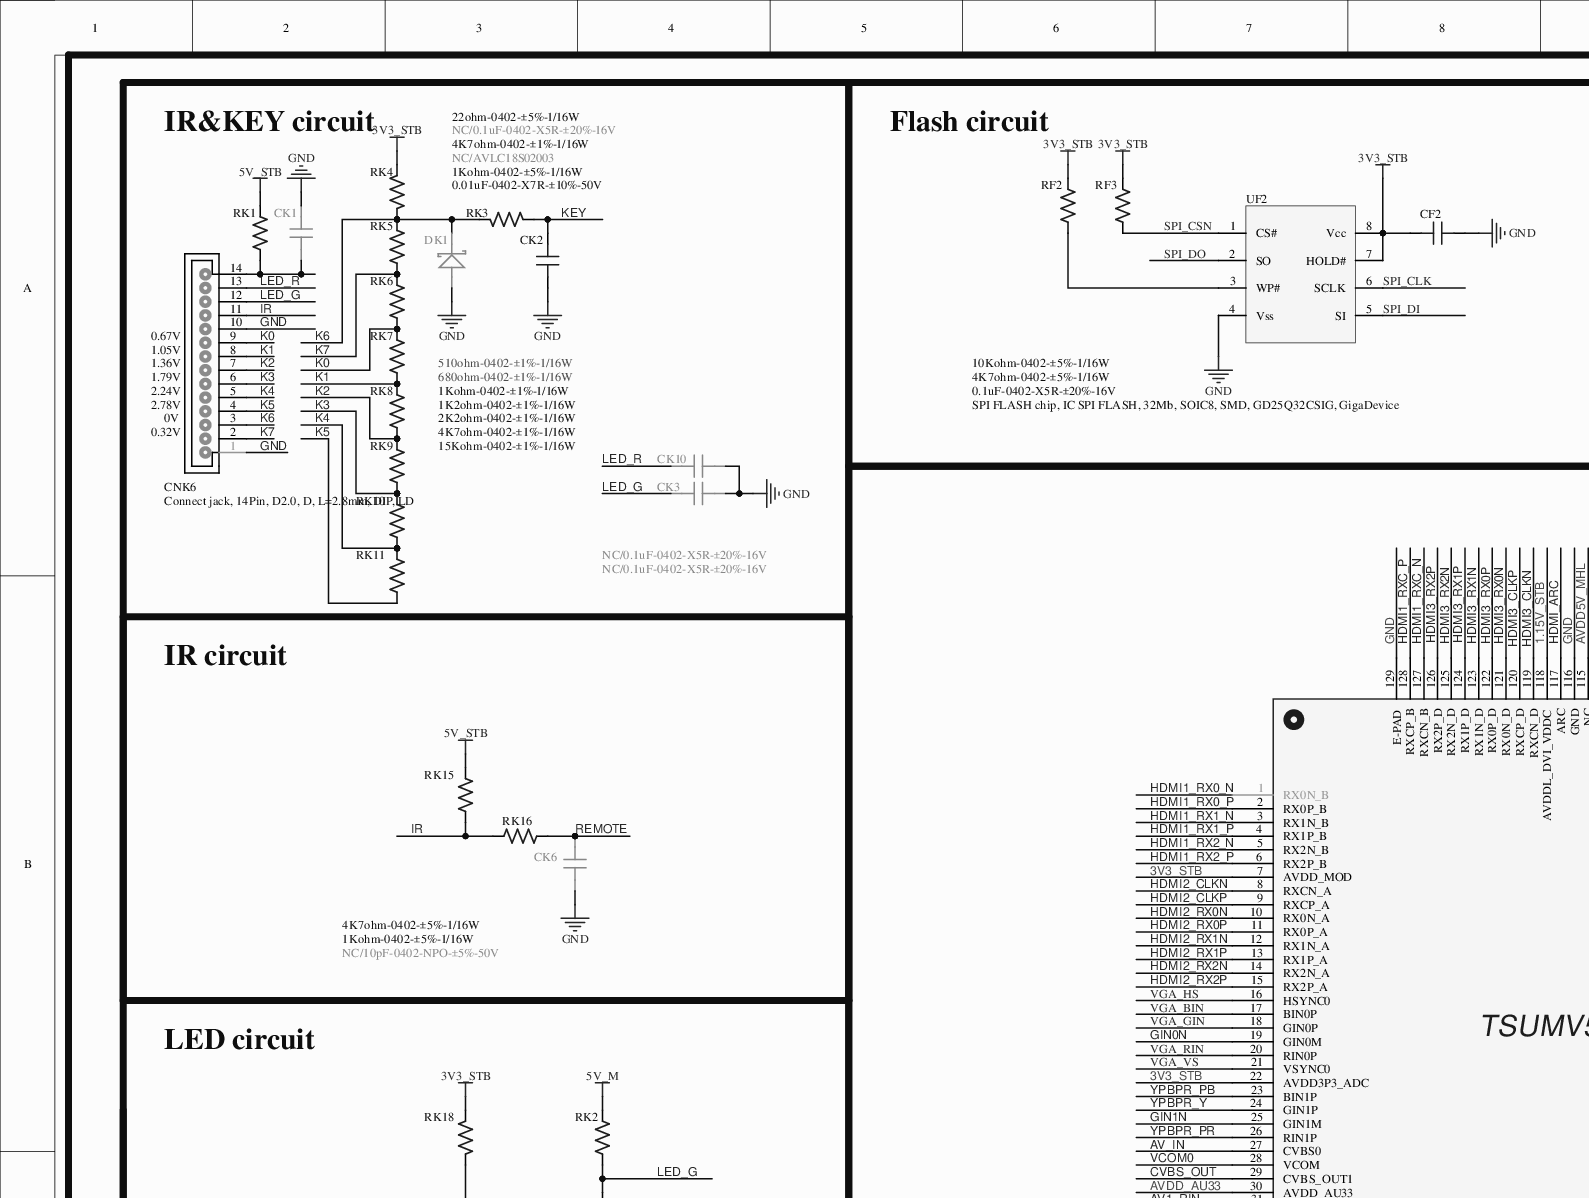
[diagram p0: MISC84277-8.SchDoc, top left]
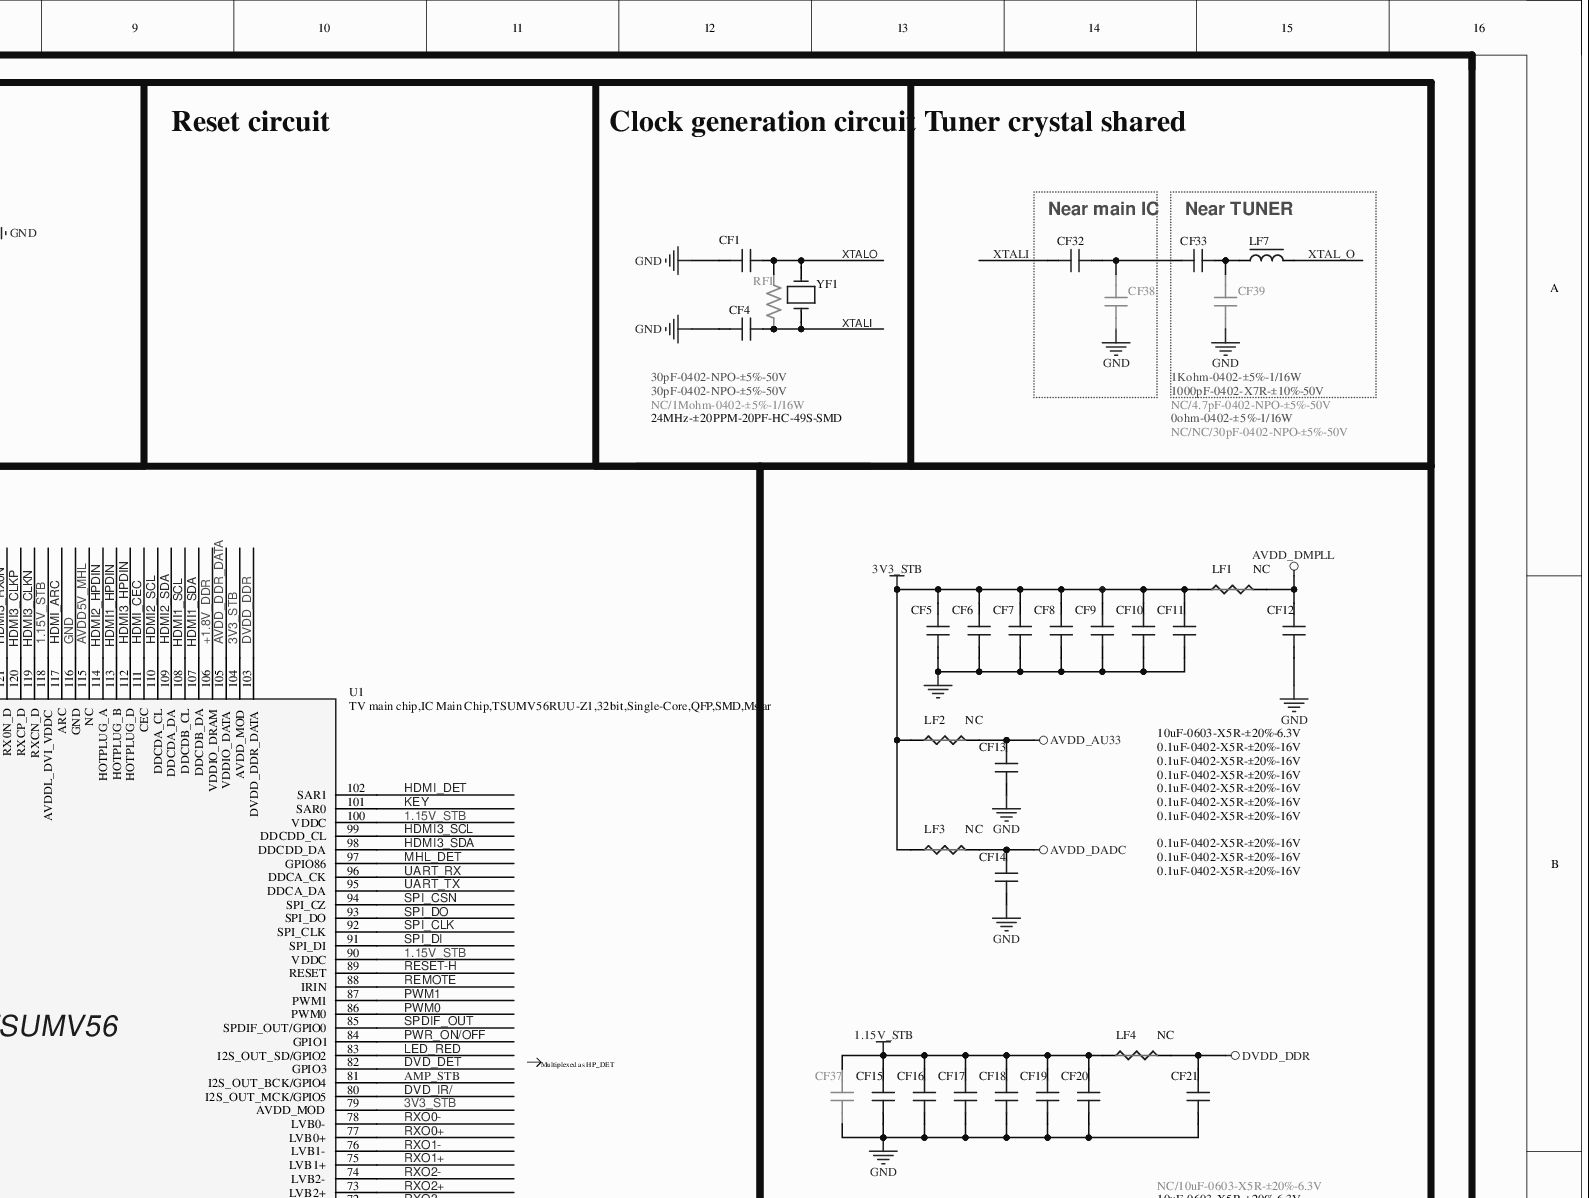
[diagram p1: MISC84277-8.SchDoc, top right]
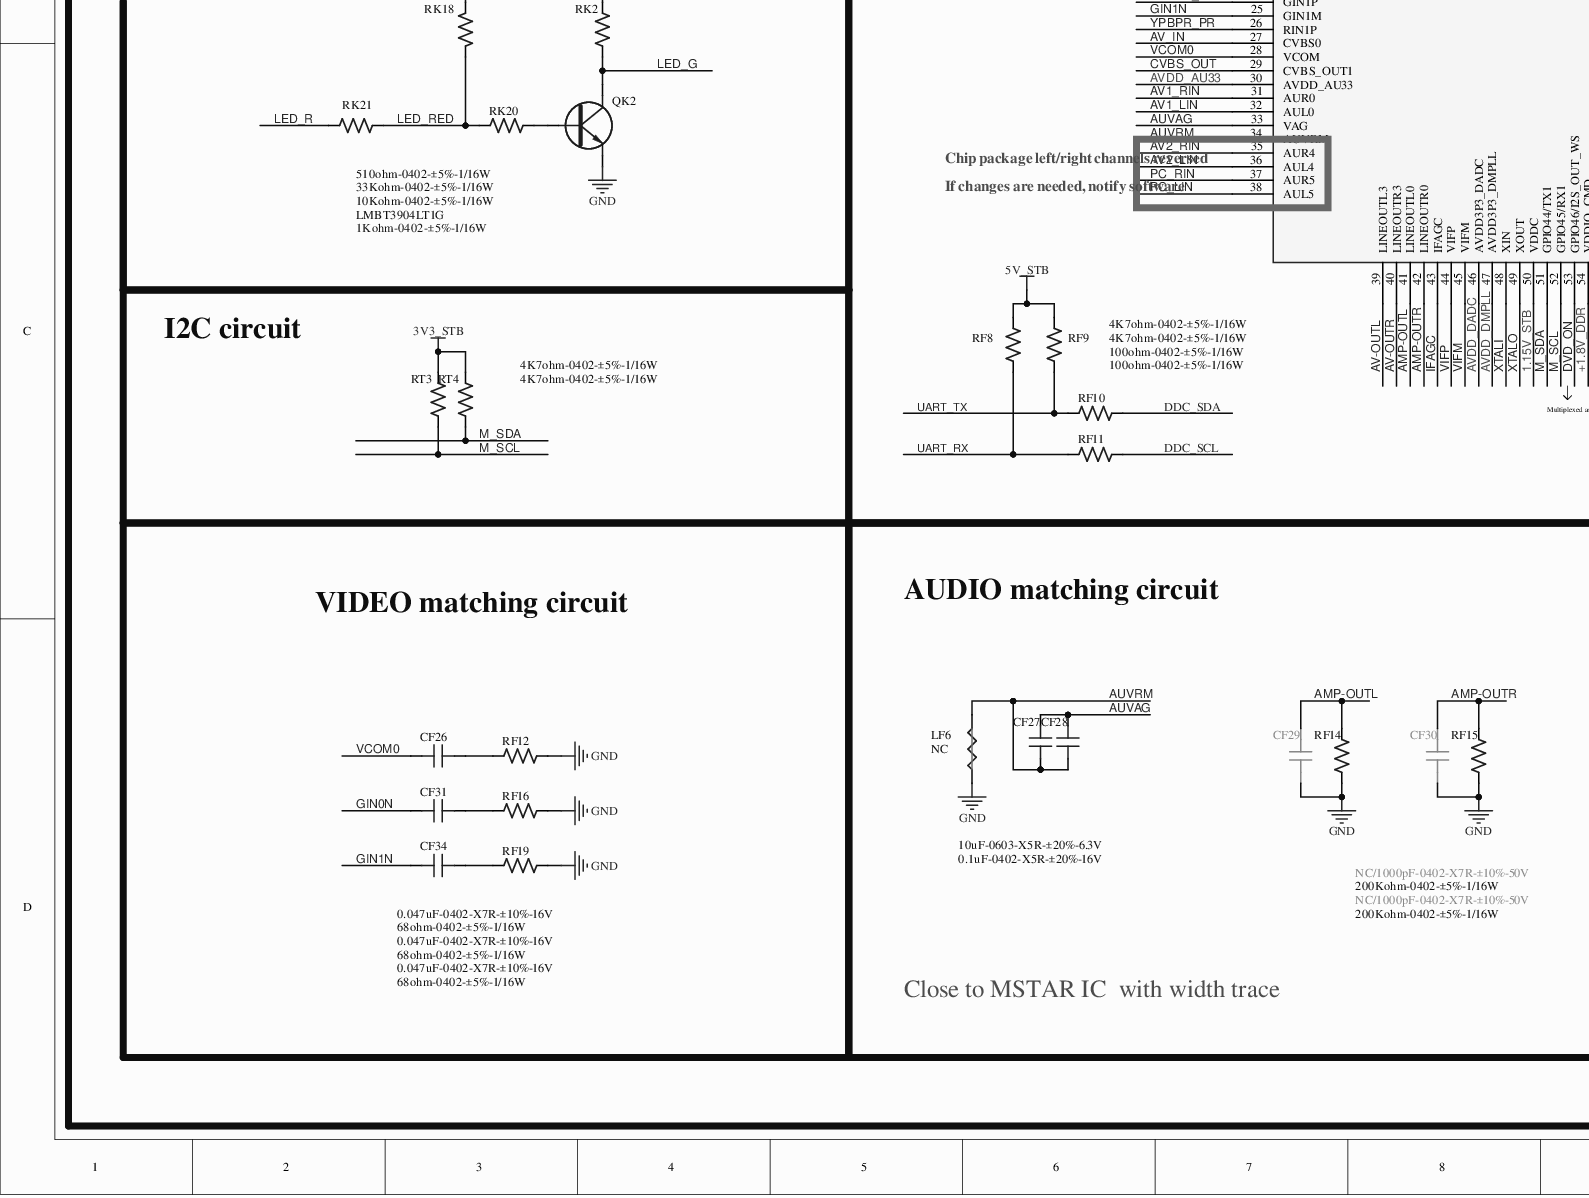
[diagram p2: MISC84277-8.SchDoc, bottom left]
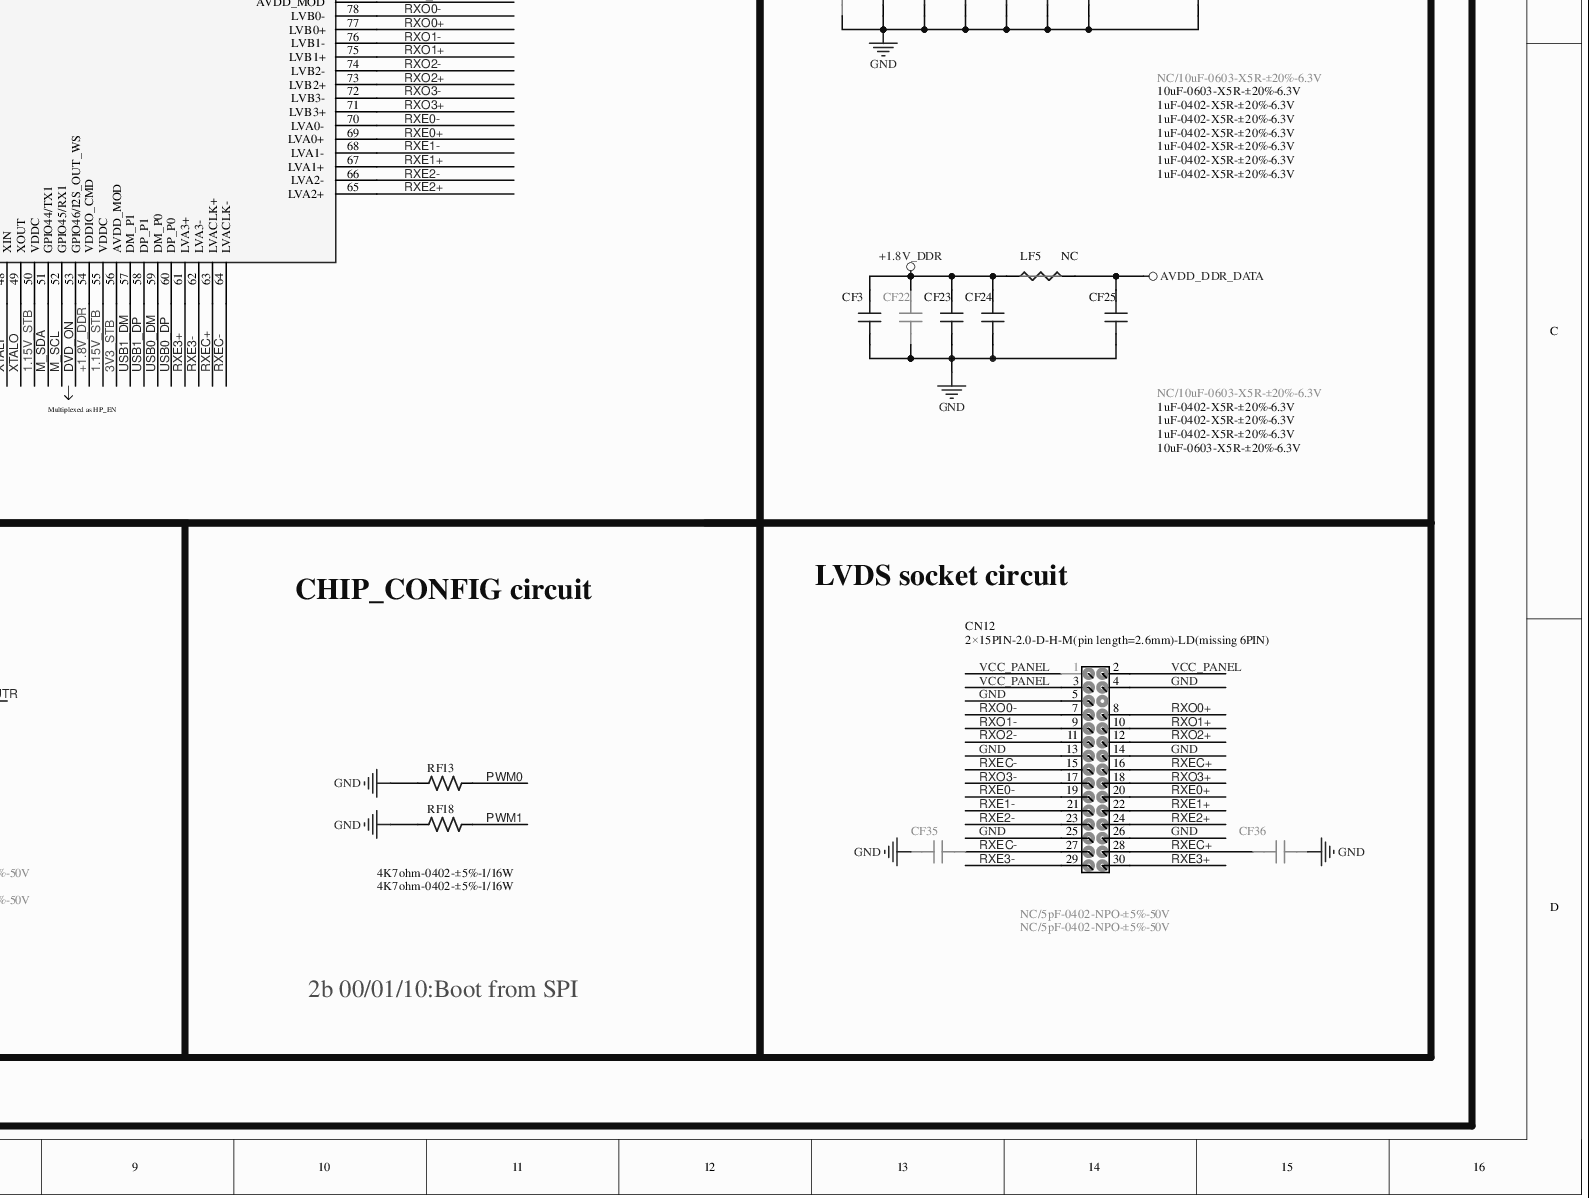
[diagram p3: MISC84277-8.SchDoc, bottom right]
# Altium project MISC84277-14.PrjPCB (part 7 of 10)

## Sheet MISC84277-8.SchDoc
size 571 x 426 mm

### Parts
CF1  30pF-0402-NPO-±5%-50V  [C0402]
CF2  0.1uF-0402-X5R-±20%-16V  [C0402]
CF3  10uF-0603-X5R-±20%-6.3V  [C0603]
CF4  30pF-0402-NPO-±5%-50V  [C0402]
CF5  10uF-0603-X5R-±20%-6.3V  [C0603]
CF6  0.1uF-0402-X5R-±20%-16V  [C0402]
CF7  0.1uF-0402-X5R-±20%-16V  [C0402]
CF8  0.1uF-0402-X5R-±20%-16V  [C0402]
CF9  0.1uF-0402-X5R-±20%-16V  [C0402]
CF10  0.1uF-0402-X5R-±20%-16V  [C0402]
CF11  0.1uF-0402-X5R-±20%-16V  [C0402]
CF12  0.1uF-0402-X5R-±20%-16V  [C0402]
CF13  0.1uF-0402-X5R-±20%-16V  [C0402]
CF14  0.1uF-0402-X5R-±20%-16V  [C0402]
CF15  10uF-0603-X5R-±20%-6.3V  [C0603]
CF16  1uF-0402-X5R-±20%-6.3V  [C0402]
CF17  1uF-0402-X5R-±20%-6.3V  [C0402]
CF18  1uF-0402-X5R-±20%-6.3V  [C0402]
CF19  1uF-0402-X5R-±20%-6.3V  [C0402]
CF20  1uF-0402-X5R-±20%-6.3V  [C0402]
CF21  1uF-0402-X5R-±20%-6.3V  [C0402]
CF22  NC/10uF-0603-X5R-±20%-6.3V  [C0603]
CF23  1uF-0402-X5R-±20%-6.3V  [C0402]
CF24  1uF-0402-X5R-±20%-6.3V  [C0402]
CF25  1uF-0402-X5R-±20%-6.3V  [C0402]
CF26  0.047uF-0402-X7R-±10%-16V  [C0402]
CF27  0.1uF-0402-X5R-±20%-16V  [C0402]
CF28  10uF-0603-X5R-±20%-6.3V  [C0603]
CF29  NC/1000pF-0402-X7R-±10%-50V  [C0402]
CF30  NC/1000pF-0402-X7R-±10%-50V  [C0402]
CF31  0.047uF-0402-X7R-±10%-16V  [C0402]
CF32  1Kohm-0402-±5%-1/16W  [C0402]
CF33  1000pF-0402-X7R-±10%-50V  [C0402]
CF34  0.047uF-0402-X7R-±10%-16V  [C0402]
CF35  NC/5pF-0402-NPO-±5%-50V  [C0402]
CF36  NC/5pF-0402-NPO-±5%-50V  [C0402]
CF37  NC/10uF-0603-X5R-±20%-6.3V  [C0603]
CF38  NC/NC/30pF-0402-NPO-±5%-50V  [C0402]
CF39  NC/4.7pF-0402-NPO-±5%-50V  [C0402]
CK1  NC/0.1uF-0402-X5R-±20%-16V  [C0402]
CK2  0.01uF-0402-X7R-±10%-50V  [C0402]
CK3  NC/0.1uF-0402-X5R-±20%-16V  [C0402]
CK6  NC/10pF-0402-NPO-±5%-50V  [C0402]
CK10  NC/0.1uF-0402-X5R-±20%-16V  [C0402]
CN12  2×15PIN-2.0-D-H-M(pin length=2.6mm)-LD(missing 6PIN)  [SIP2*15/2.0D-2]
CNK6  Connect jack, 14Pin, D2.0, D, L=2.8mm, DIP, LD  [SIP14/2.0D-1]
DK1  NC/AVLC18S02003  [DIODE-S0402]
LF1  NC  [GND]
LF2  NC  [GND]
LF3  NC  [GND]
LF4  NC  [GND]
LF5  NC  [GND]
LF6  NC  [GND]
LF7  0ohm-0402-±5%-1/16W  [L0402]
QK2  LMBT3904LT1G  [SOT-23]
RF1  NC/1Mohm-0402-±5%-1/16W  [R0402]
RF2  10Kohm-0402-±5%-1/16W  [R0402]
RF3  4K7ohm-0402-±5%-1/16W  [R0402]
RF8  4K7ohm-0402-±5%-1/16W  [R0402]
RF9  4K7ohm-0402-±5%-1/16W  [R0402]
RF10  100ohm-0402-±5%-1/16W  [R0402]
RF11  100ohm-0402-±5%-1/16W  [R0402]
RF12  68ohm-0402-±5%-1/16W  [R0402]
RF13  4K7ohm-0402-±5%-1/16W  [R0402]
RF14  200Kohm-0402-±5%-1/16W  [R0402]
RF15  200Kohm-0402-±5%-1/16W  [R0402]
RF16  68ohm-0402-±5%-1/16W  [R0402]
RF18  4K7ohm-0402-±5%-1/16W  [R0402]
RF19  68ohm-0402-±5%-1/16W  [R0402]
RK1  22ohm-0402-±5%-1/16W  [R0402]
RK2  1Kohm-0402-±5%-1/16W  [R0402]
RK3  1Kohm-0402-±5%-1/16W  [R0402]
RK4  4K7ohm-0402-±1%-1/16W  [R0402]
RK5  510ohm-0402-±1%-1/16W  [R0402]
RK6  680ohm-0402-±1%-1/16W  [R0402]
RK7  1Kohm-0402-±1%-1/16W  [R0402]
RK8  1K2ohm-0402-±1%-1/16W  [R0402]
RK9  2K2ohm-0402-±1%-1/16W  [R0402]
RK10  4K7ohm-0402-±1%-1/16W  [R0402]
RK11  15Kohm-0402-±1%-1/16W  [R0402]
RK15  4K7ohm-0402-±5%-1/16W  [R0402]
RK16  1Kohm-0402-±5%-1/16W  [R0402]
RK18  33Kohm-0402-±5%-1/16W  [R0402]
RK20  10Kohm-0402-±5%-1/16W  [R0402]
RK21  510ohm-0402-±5%-1/16W  [R0402]
RT3  4K7ohm-0402-±5%-1/16W  [R0402]
RT4  4K7ohm-0402-±5%-1/16W  [R0402]
U1  TV main chip,IC Main Chip,TSUMV56RUU-Z1,32bit,Single-Core,QFP,SMD,Mstar  [QFP128/0.4-5]
UF2  SPI FLASH chip, IC SPI FLASH, 32Mb, SOIC8, SMD, GD25Q32CSIG, GigaDevice  [SOIC8]
YF1  24MHz-±20PPM-20PF-HC-49S-SMD  [XTAL-S-1]

### Blocks framed on the sheet
Flash circuit: CF2 RF2 RF3 UF2
Near main IC: CF32 CF38
Near TUNER: CF33 CF39 LF7
VIDEO matching circuit: CF26 CF31 CF34 RF12 RF16 RF19
AUDIO matching circuit: CF27-CF30 LF6 RF14 RF15
CHIP_CONFIG circuit: RF13 RF18

### Nets
1.15V_STB: CF15.1 CF16.2 CF17.2 CF18.2 CF19.2 CF20.2 CF37.1 LF4.JP_2K U1.50(VDDC) U1.55(VDDC) U1.90(VDDC) U1.100(VDDC) U1.118(AVDDL_DVI_VDDC)
3V3_STB: CF2.2 CF5.1 CF6.2 CF7.2 CF8.2 CF9.2 CF10.2 CF11.2 LF1.JP_2K LF2.JP_2K LF3.JP_2K RF2.2 RF3.2 RK4.2 RK18.2 RT3.1 RT4.1 U1.7(AVDD_MOD) U1.22(AVDD3P3_ADC) U1.56(AVDD_MOD) U1.79(AVDD_MOD) U1.104(AVDD_MOD) UF2.7(HOLD#) UF2.8(Vcc)
5V_M: RK2.2
5V_STB: RF8.2 RF9.2 RK1.1 RK15.1
+1.8V_DDR: CF3.1 CF22.1 CF23.2 CF24.2 LF5.JP_2K U1.54(VDDIO_CMD) U1.106(VDDIO_DRAM)
AVDD_AU33: CF13.2 LF2.JP_1K U1.30(AVDD_AU33)
AVDD_DADC: CF14.2 LF3.JP_1K U1.46(AVDD3P3_DADC)
AVDD_DDR_DATA: CF25.2 LF5.JP_1K U1.105(VDDIO_DATA)
AVDD_DMPLL: CF12.2 LF1.JP_1K U1.47(AVDD3P3_DMPLL)
DVDD_DDR: CF21.2 LF4.JP_1K U1.103(DVDD_DDR_DATA)
GND: CF1.1 CF2.1 CF3.2 CF4.1 CF5.2 CF6.1 CF7.1 CF8.1 CF9.1 CF10.1 CF11.1 CF12.1 CF13.1 CF14.1 CF15.2 CF16.1 CF17.1 CF18.1 CF19.1 CF20.1 CF21.1 CF22.2 CF23.1 CF24.1 CF25.1 CF29.2 CF30.2 CF35.1 CF36.2 CF37.2 CF38.1 CF39.1 CK1.1 CK2.2 CK3.1 CK6.1 CK10.1 CN12.4 CN12.5 CN12.13 CN12.14 CN12.25 CN12.26 CNK6.1 CNK6.10 DK1.A LF6.JP_2K QK2.E RF12.2 RF13.2 RF14.1 RF15.1 RF16.2 RF18.2 RF19.2 U1.116(GND) U1.129(E-PAD) UF2.4(Vss)
VCC_PANEL: CN12.1 CN12.2 CN12.3
AMP-OUTL: CF29.1 RF14.2 U1.41(LINEOUTL0)
AMP-OUTR: CF30.1 RF15.2 U1.42(LINEOUTR0)
AMP_STB: U1.81(I2S_OUT_BCK/GPIO4)
AUVAG: CF27.2 CF28.1 U1.33(VAG)
AUVRM: CF27.1 CF28.2 LF6.JP_1K U1.34(AUVRM)
AV1_LIN: U1.32(AUL0)
AV1_RIN: U1.31(AUR0)
AV2_LIN: U1.36(AUL4)
AV2_RIN: U1.35(AUR4)
AV-OUTL: U1.39(LINEOUTL3)
AV-OUTR: U1.40(LINEOUTR3)
AV_IN: U1.27(CVBS0)
AVDD5V_MHL: U1.115(NC)
CVBS_OUT: U1.29(CVBS_OUT1)
DDC_SCL: RF11.2
DDC_SDA: RF10.2
DVD_DET: U1.82(GPIO3)
DVD_IR/: U1.80(I2S_OUT_MCK/GPIO5)
DVD_ON: U1.53(GPIO46/I2S_OUT_WS)
GIN0N: CF31.1 U1.19(GIN0M)
GIN1N: CF34.1 U1.25(GIN1M)
HDMI1_HPDIN: U1.113(HOTPLUG_B)
HDMI1_RX0_N: U1.1(RX0N_B)
HDMI1_RX0_P: U1.2(RX0P_B)
HDMI1_RX1_N: U1.3(RX1N_B)
HDMI1_RX1_P: U1.4(RX1P_B)
HDMI1_RX2_N: U1.5(RX2N_B)
HDMI1_RX2_P: U1.6(RX2P_B)
HDMI1_RXC_N: U1.127(RXCN_B)
HDMI1_RXC_P: U1.128(RXCP_B)
HDMI1_SCL: U1.108(DDCDB_CL)
HDMI1_SDA: U1.107(DDCDB_DA)
HDMI2_CLKN: U1.8(RXCN_A)
HDMI2_CLKP: U1.9(RXCP_A)
HDMI2_HPDIN: U1.114(HOTPLUG_A)
HDMI2_RX0N: U1.10(RX0N_A)
HDMI2_RX0P: U1.11(RX0P_A)
HDMI2_RX1N: U1.12(RX1N_A)
HDMI2_RX1P: U1.13(RX1P_A)
HDMI2_RX2N: U1.14(RX2N_A)
HDMI2_RX2P: U1.15(RX2P_A)
HDMI2_SCL: U1.110(DDCDA_CL)
HDMI2_SDA: U1.109(DDCDA_DA)
HDMI3_CLKN: U1.119(RXCN_D)
HDMI3_CLKP: U1.120(RXCP_D)
HDMI3_HPDIN: U1.112(HOTPLUG_D)
HDMI3_RX0N: U1.121(RX0N_D)
HDMI3_RX0P: U1.122(RX0P_D)
HDMI3_RX1N: U1.123(RX1N_D)
HDMI3_RX1P: U1.124(RX1P_D)
HDMI3_RX2N: U1.125(RX2N_D)
HDMI3_RX2P: U1.126(RX2P_D)
HDMI3_SCL: U1.99(DDCDD_CL)
HDMI3_SDA: U1.98(DDCDD_DA)
HDMI_ARC: U1.117(ARC)
HDMI_CEC: U1.111(CEC)
HDMI_DET: U1.102(SAR1)
IFAGC: U1.43(IFAGC)
IR: CNK6.11 RK15.2 RK16.2
K0: CNK6.9 RK6.1 RK7.1
K1: CNK6.8 RK7.2 RK8.1
K2: CNK6.7 RK8.2 RK9.1
K3: CNK6.6 RK9.2 RK10.1
K4: CNK6.5 RK10.2 RK11.1
K5: CNK6.4 RK11.2
K6: CNK6.3 DK1.K RK3.2 RK4.1 RK5.1
K7: CNK6.2 RK5.2 RK6.2
KEY: CK2.1 RK3.1 U1.101(SAR0)
LED_G: CK3.2 CNK6.12 QK2.C RK2.1
LED_R: CK10.2 CNK6.13 RK21.2
LED_RED: RK18.1 RK20.2 RK21.1 U1.83(I2S_OUT_SD/GPIO2)
M_SCL: RT3.2 U1.52(GPIO45/RX1)
M_SDA: RT4.2 U1.51(GPIO44/TX1)
MHL_DET: U1.97(GPIO86)
PC_LIN: U1.38(AUL5)
PC_RIN: U1.37(AUR5)
PWM0: RF13.1 U1.86(PWM0)
PWM1: RF18.1 U1.87(PWM1)
PWR_ON/OFF: U1.84(GPIO1)
REMOTE: CK6.2 RK16.1 U1.88(IRIN)
RESET-H: U1.89(RESET)
RXE0+: CN12.20 U1.69(LVA0+)
RXE0-: CN12.19 U1.70(LVA0-)
RXE1+: CN12.22 U1.67(LVA1+)
RXE1-: CN12.21 U1.68(LVA1-)
RXE2+: CN12.24 U1.65(LVA2+)
RXE2-: CN12.23 U1.66(LVA2-)
RXE3+: CN12.30 U1.61(LVA3+)
RXE3-: CN12.29 U1.62(LVA3-)
RXEC+: CF36.1 CN12.16 CN12.28 U1.63(LVACLK+)
RXEC-: CF35.2 CN12.15 CN12.27 U1.64(LVACLK-)
RXO0+: CN12.8 U1.77(LVB0+)
RXO0-: CN12.7 U1.78(LVB0-)
RXO1+: CN12.10 U1.75(LVB1+)
RXO1-: CN12.9 U1.76(LVB1-)
RXO2+: CN12.12 U1.73(LVB2+)
RXO2-: CN12.11 U1.74(LVB2-)
RXO3+: CN12.18 U1.71(LVB3+)
RXO3-: CN12.17 U1.72(LVB3-)
SPDIF_OUT: U1.85(SPDIF_OUT/GPIO0)
SPI_CLK: U1.92(SPI_CLK) UF2.6(SCLK)
SPI_CSN: RF3.1 U1.94(SPI_CZ) UF2.1(CS#)
SPI_DI: U1.91(SPI_DI) UF2.5(SI)
SPI_DO: U1.93(SPI_DO) UF2.2(SO)
UART_RX: RF8.1 RF11.1 U1.96(DDCA_CK)
UART_TX: RF9.1 RF10.1 U1.95(DDCA_DA)
USB0_DM: U1.59(DM_P0)
USB0_DP: U1.60(DP_P0)
USB1_DM: U1.57(DM_P1)
USB1_DP: U1.58(DP_P1)
VCOM0: CF26.1 U1.28(VCOM)
VGA_BIN: U1.17(BIN0P)
VGA_GIN: U1.18(GIN0P)
VGA_HS: U1.16(HSYNC0)
VGA_RIN: U1.20(RIN0P)
VGA_VS: U1.21(VSYNC0)
VIFM: U1.45(VIFM)
VIFP: U1.44(VIFP)
XTAL_O: LF7.2
XTALI: CF4.2 CF32.2 RF1.1 U1.48(XIN) YF1.1
XTALO: CF1.2 RF1.2 U1.49(XOUT) YF1.2
YPBPR_PB: U1.23(BIN1P)
YPBPR_PR: U1.26(RIN1P)
YPBPR_Y: U1.24(GIN1P)
NetCF26_2: CF26.2 RF12.1
NetCF31_2: CF31.2 RF16.1
NetCF32_1: CF32.1 CF33.2 CF38.2
NetCF33_1: CF33.1 CF39.2 LF7.1
NetCF34_2: CF34.2 RF19.1
NetCK1_2: CK1.2 CNK6.14 RK1.2
NetQK2_B: QK2.B RK20.1
NetRF2_1: RF2.1 UF2.3(WP#)

### Notes on the sheet
- (near RK4) IR&KEY circuit
- Reset circuit
- Clock generation circuit
- Tuner crystal shared
- (near CNK6) 0.67V
- (near CNK6) 1.05V
- (near CNK6) 1.36V
- (near CNK6) 1.79V
- (near CNK6) 2.24V
- (near CNK6) 2.78V
- (near CNK6) 0.32V
- (near CNK6) 0V
- IR circuit
- LED circuit
- Multiplexed as HP_DET
- (near U1) Chip package left/right channels reversed
- (near U1) If changes are needed, notify software
- I2C circuit
- Multiplexed as HP_EN
- LVDS socket circuit
- Close to MSTAR IC  with width trace
- 2b 00/01/10:Boot from SPI

### Library data of the parts
CF1 CF32 CF38 CF39 = 30pF-0402-NPO-±5%-50V-D
CF2 CF7-CF10 CF12-CF14 CF17 CF27 CK1 CK3 CK10 = 0.1uF-0402-Y5V-+80%-20%-16V-D
CF3 CF5 CF15 CF22 CF28 CF37 = 10uF-0603-X5R-±20%-6.3V-D
CF4 = 33pF-0402-NPO-±5%-50V-D
CF6 CF11 CF16 CF18-CF21 CF23-CF25 = 1uF-0402-X5R-±20%-6.3V-D
CF26 CF31 CF34 = 0.047uF-0402-X7R-±10%-16V-D
CF29 CF30 CF33 = 1000pF-0402-X7R-±10%-50V-D
CF35 CF36 = 5pF-0402-NPO-±5%-50V-D
CK2 = 0.01uF-0402-X7R-±10%-50V-D
CK6 = 10pF-0402-NPO-±5%-50V-D
CN12 = 2×15PIN-2.0-D-H-M(脚长=2.6mm)(缺6PIN)-LD-DHMI: CN-straight gold pin
CNK6 = 14PIN-2.0-D-H-G-DHMI
DK1 = AVLC18S02003-D
LF1-LF6 = GND: Manufacturer: Panasonic; Part Number: ERJ3GEYJ473V; Right: 20; Bottom: 30; CLASS: Discrete; Comments: Digikey
LF7 = SDCL1005CR33JTDF-D
QK2 = MMBT3904(f≥350MHz)-D-NPN: Q-NPN-#-#-#
RF1 = 1Mohm-0402-±5%-1/16W-D
RF2 RK20 = 10Kohm-0402-±5%-1/16W-D
RF3 RF8 RF9 RF13 RF18 RK15 RK18 RT3 RT4 = 4K7ohm-0402-±5%-1/16W-D
RF10 RF11 = 100ohm-0402-±5%-1/16W-D
RF12 RF16 RF19 = 68ohm-0402-±5%-1/16W-D
RF14 RF15 = 200Kohm-0402-±5%-1/16W-D
RK1 = 22ohm-0402-±5%-1/16W-D
RK2 RK3 RK16 RK21 = 1Kohm-0402-±5%-1/16W-D
RK4 = 4K7ohm-0402-±1%-1/16W-D
RK5 = 2K2ohm-0402-±5%-1/16W-D
RK6 = 680ohm-0402-±5%-1/16W-D
RK7 = 5K6ohm-0402-±1%-1/16W-D
RK8 = 10Kohm-0402-±1%-1/16W-D
RK9 = 20Kohm-0402-±1%-1/16W-D
RK10 = 0ohm-0402-±5%-1/16W-D
RK11 = 1K2ohm-0402-±5%-1/16W-D
U1 = TSU69ZR-D
UF2 = SPI FLASH 芯片,IC SPI FLASH,32Mb,SOIC8,SMD,GD25Q32CSIG,GigaDevice-D
YF1 = 24MHz-±20PPM-20PF-HC-49S-SMD-D